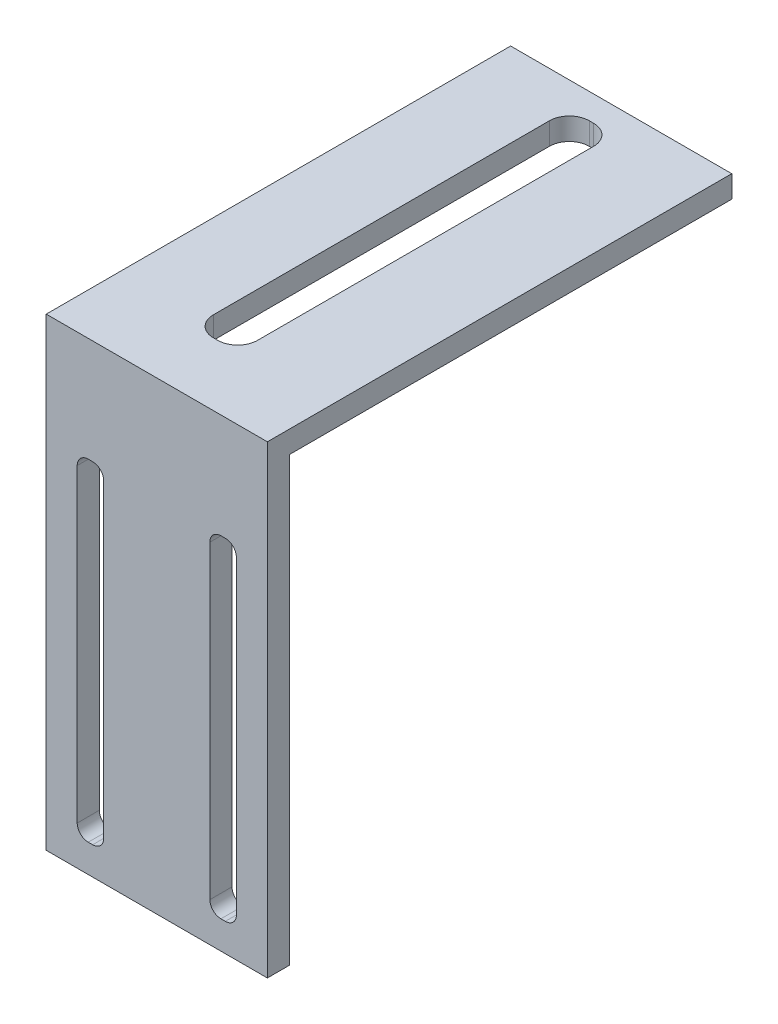
from build123d import *

# Parameters (mm, degrees)
SKETCH1_W                = 50
SKETCH1_H                = 100
BOSS_EXTRUDE1_DEPTH      = 5
CUT_EXTRUDE1_DEPTH       = 10
BOSS_EXTRUDE2_DEPTH      = 100
BOSS_EXTRUDE2_DEPTH_BACK = 5
SKETCH4_W                = 50
SKETCH4_H                = 5
CUT_EXTRUDE3_DEPTH       = 80


with BuildPart() as part:
    # Sketch1 → Boss-Extrude1 (new body)
    with BuildSketch(Plane.XY):
        Rectangle(SKETCH1_W, SKETCH1_H)
    extrude(amount=BOSS_EXTRUDE1_DEPTH)

    # Sketch2 → Cut-Extrude1 (cut)
    with BuildSketch(Plane.XY.offset(5)):
        with BuildLine():
            Line((-14.5, -43.655057898), (-15.5, -43.655057898))
            ThreePointArc((-15.5, -43.655057898), (-17.267766953, -42.922824851), (-18, -41.155057898))
            Line((-18, -41.155057898), (-18, 28.844942102))
            ThreePointArc((-18, 28.844942102), (-17.267766953, 30.612709055), (-15.5, 31.344942102))
            Line((-15.5, 31.344942102), (-14.5, 31.344942102))
            ThreePointArc((-14.5, 31.344942102), (-12.732233047, 30.612709055), (-12, 28.844942102))
            Line((-12, 28.844942102), (-12, -41.155057898))
            ThreePointArc((-12, -41.155057898), (-12.732233047, -42.922824851), (-14.5, -43.655057898))
        make_face()
        with BuildLine():
            Line((15.5, -43.655057898), (14.5, -43.655057898))
            ThreePointArc((14.5, -43.655057898), (12.732233047, -42.922824851), (12, -41.155057898))
            Line((12, -41.155057898), (12, 28.844942102))
            ThreePointArc((12, 28.844942102), (12.732233047, 30.612709055), (14.5, 31.344942102))
            Line((14.5, 31.344942102), (15.5, 31.344942102))
            ThreePointArc((15.5, 31.344942102), (17.267766953, 30.612709055), (18, 28.844942102))
            Line((18, 28.844942102), (18, -41.155057898))
            ThreePointArc((18, -41.155057898), (17.267766953, -42.922824851), (15.5, -43.655057898))
        make_face()
    extrude(amount=-CUT_EXTRUDE1_DEPTH, mode=Mode.SUBTRACT)

    # Sketch4 → Boss-Extrude2 (add, two sides: drawn at the far end of the back side and taken through both)
    with BuildSketch(Plane(origin=(0, 0, 0), x_dir=(-1, 0, 0), z_dir=(0, 0, -1)).offset(-BOSS_EXTRUDE2_DEPTH_BACK)):
        with Locations((0, 52.5)):
            Rectangle(SKETCH4_W, SKETCH4_H)
    extrude(amount=BOSS_EXTRUDE2_DEPTH + BOSS_EXTRUDE2_DEPTH_BACK)

    # Sketch5 → Cut-Extrude3 (cut)
    with BuildSketch(Plane.XZ.offset(-50)):
        with BuildLine():
            Line((-0.473985761, -94.252877225), (-1.473985761, -94.252877225))
            ThreePointArc((-1.473985761, -94.252877225), (-4.655966276, -92.934857741), (-5.973985761, -89.752877225))
            Line((-5.973985761, -89.752877225), (-5.973985761, -13.752877225))
            ThreePointArc((-5.973985761, -13.752877225), (-4.655966276, -10.57089671), (-1.473985761, -9.252877225))
            Line((-1.473985761, -9.252877225), (-0.473985761, -9.252877225))
            ThreePointArc((-0.473985761, -9.252877225), (2.707994755, -10.57089671), (4.026014239, -13.752877225))
            Line((4.026014239, -13.752877225), (4.026014239, -89.752877225))
            ThreePointArc((4.026014239, -89.752877225), (2.707994755, -92.934857741), (-0.473985761, -94.252877225))
        make_face()
    extrude(amount=-CUT_EXTRUDE3_DEPTH, mode=Mode.SUBTRACT)


solid = part.part
